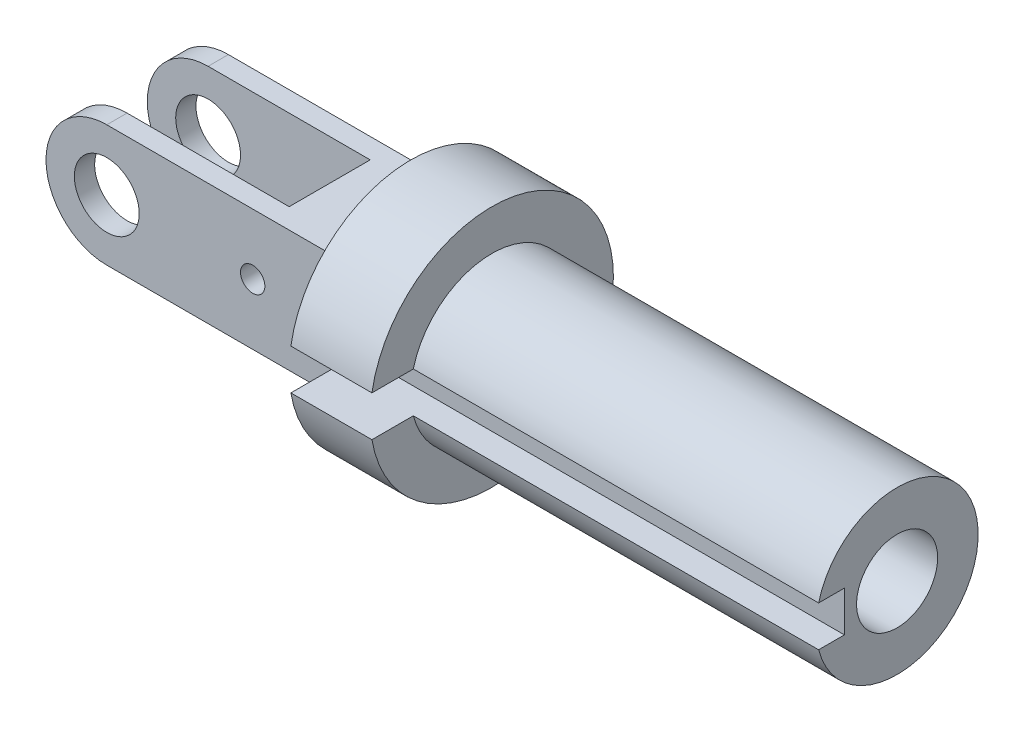
from build123d import *

# Parameters (mm, degrees)
SKETCH2_R           = 0.4
BOSS_EXTRUDE1_DEPTH = 0.75
CUT_EXTRUDE1_DEPTH  = 0.5
SKETCH4_R           = 0.5
CUT_EXTRUDE2_DEPTH  = 6
CUT_EXTRUDE4_DEPTH  = 6
SKETCH6_R           = 0.15
CUT_EXTRUDE5_DEPTH  = 1


with BuildPart() as part:
    # Sketch1 → Revolve1 (revolve)
    with BuildSketch(Plane.XY, mode=Mode.PRIVATE) as revolve1_sk:
        Polygon((0, 0), (0, 1.5), (1, 1.5), (1, 1), (6, 1), (6, 0), align=None)
    revolve(revolve1_sk.sketch.rotate(Axis((0.124352332, 0, 0), (1, 0, 0)), 90), axis=Axis((0.124352332, 0, 0), (1, 0, 0)))

    # Sketch2 → Boss-Extrude1 (add, symmetric)
    with BuildSketch(Plane.XY):
        with BuildLine():
            Line((0, 0.75), (0, -0.75))
            Line((0, -0.75), (-3, -0.75))
            ThreePointArc((-3, -0.75), (-3.75, 0), (-3, 0.75))
            Line((-3, 0.75), (0, 0.75))
        make_face()
        with Locations((-3, 0)):
            Circle(SKETCH2_R, mode=Mode.SUBTRACT)
    extrude(amount=BOSS_EXTRUDE1_DEPTH, both=True)

    # Sketch3 → Cut-Extrude1 (cut, symmetric)
    with BuildSketch(Plane.XY):
        with BuildLine():
            Line((-1, 0.75), (-1, -0.75))
            Line((-1, -0.75), (-3, -0.75))
            ThreePointArc((-3, -0.75), (-3.75, 0), (-3, 0.75))
            Line((-3, 0.75), (-1, 0.75))
        make_face()
    extrude(amount=CUT_EXTRUDE1_DEPTH, both=True, mode=Mode.SUBTRACT)

    # Sketch4 → Cut-Extrude2 (cut)
    with BuildSketch(Plane(origin=(6, 0, 0), x_dir=(0, 0, -1), z_dir=(1, 0, 0))):
        Circle(SKETCH4_R)
    extrude(amount=-CUT_EXTRUDE2_DEPTH, mode=Mode.SUBTRACT)

    # Sketch5 → Cut-Extrude4 (cut)
    with BuildSketch(Plane(origin=(6, 0, 0), x_dir=(0, 0, -1), z_dir=(1, 0, 0))):
        with BuildLine():
            Line((-0.65, -0.25), (-0.65, 0.25))
            Line((-0.65, 0.25), (-0.968245837, 0.25))
            ThreePointArc((-0.968245837, 0.25), (-1, 0), (-0.968245837, -0.25))
            Line((-0.968245837, -0.25), (-0.65, -0.25))
        make_face()
        with BuildLine():
            ThreePointArc((-0.968245837, -0.25), (-1, 0), (-0.968245837, 0.25))
            Line((-0.968245837, 0.25), (-1.818815546, 0.25))
            Line((-1.818815546, 0.25), (-1.818815546, -0.25))
            Line((-1.818815546, -0.25), (-0.968245837, -0.25))
        make_face()
    extrude(amount=-CUT_EXTRUDE4_DEPTH, mode=Mode.SUBTRACT)

    # Sketch6 → Cut-Extrude5 (cut)
    with BuildSketch(Plane.XY.offset(0.75)):
        with Locations((-1.2, 0)):
            Circle(SKETCH6_R)
    extrude(amount=-CUT_EXTRUDE5_DEPTH, mode=Mode.SUBTRACT)


solid = part.part
